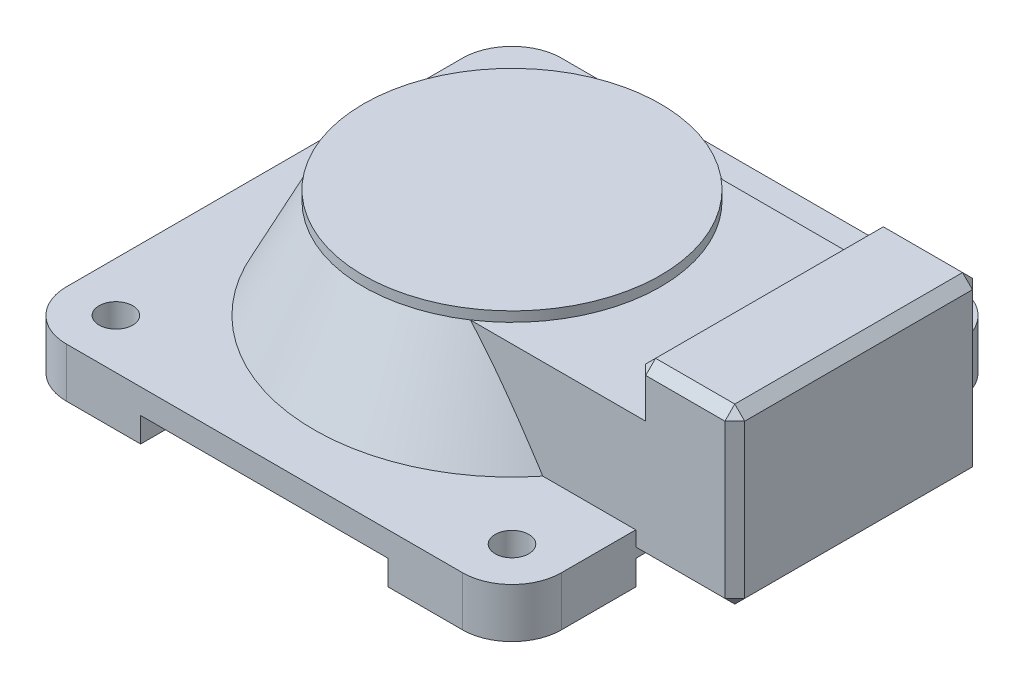
from build123d import *

# Parameters (mm, degrees)
SKETCH1_W             = 100
SKETCH1_H             = 100
BOSS_EXTRUDE1_DEPTH   = 10
SKETCH2_W             = 50
SKETCH2_H             = 10
CUT_EXTRUDE1_DEPTH    = 113.249721603
SKETCH3_W             = 50
SKETCH3_H             = 10
CUT_EXTRUDE2_DEPTH    = 113.249721603
FILLET1_R             = 10
SKETCH5_R             = 30
BOSS_EXTRUDE2_DEPTH   = 2
SKETCH6_W             = 50
SKETCH6_H             = 20
BOSS_EXTRUDE3_DEPTH   = 50
SKETCH7_W             = 50
SKETCH7_H             = 35
BOSS_EXTRUDE6_DEPTH   = 20
CHAMFER1_SIZE         = 2
M8_TAPPED_HOLE1_D     = 6.8
M8_TAPPED_HOLE1_DEPTH = 20.207073895
M8_TAPPED_HOLE1_TIP   = 2.042926105


with BuildPart() as part:
    # Sketch1 → Boss-Extrude1 (new body)
    with BuildSketch(Plane(origin=(0, 0, 0), x_dir=(1, 0, 0), z_dir=(0, 1, 0))):
        Rectangle(SKETCH1_W, SKETCH1_H)
    extrude(amount=BOSS_EXTRUDE1_DEPTH)

    # Sketch2 → Cut-Extrude1 (cut, through all)
    with BuildSketch(Plane.XY.offset(50)):
        Rectangle(SKETCH2_W, SKETCH2_H)
    extrude(amount=-CUT_EXTRUDE1_DEPTH, mode=Mode.SUBTRACT)

    # Sketch3 → Cut-Extrude2 (cut, through all)
    with BuildSketch(Plane(origin=(50, 0, 0), x_dir=(0, 0, -1), z_dir=(1, 0, 0))):
        Rectangle(SKETCH3_W, SKETCH3_H)
    extrude(amount=-CUT_EXTRUDE2_DEPTH, mode=Mode.SUBTRACT)

    # Fillet1
    fillet1_edges = [part.edges().sort_by_distance(p)[0] for p in [
        (50, 5, 50),
        (-50, 5, 50),
        (-50, 5, -50),
        (50, 5, -50),
    ]]
    fillet(fillet1_edges, radius=FILLET1_R)

    # Sketch4 → Revolve1 (revolve)
    with BuildSketch(Plane.XY):
        Polygon((0, 10), (0, 30), (30, 30), (40, 10), align=None)
    revolve(axis=Axis((0, 10, 0), (0, 1, 0)))

    # Sketch5 → Boss-Extrude2 (add)
    with BuildSketch(Plane(origin=(0, 30, 0), x_dir=(1, 0, 0), z_dir=(0, 1, 0))):
        with Locations(Location((0, 0, 0), (0, 0, 180))):
            Circle(SKETCH5_R)
    extrude(amount=BOSS_EXTRUDE2_DEPTH)

    # Sketch6 → Boss-Extrude3 (add)
    with BuildSketch(Plane(origin=(0, 0, 0), x_dir=(0, 0, -1), z_dir=(1, 0, 0))):
        with Locations((0, 20)):
            Rectangle(SKETCH6_W, SKETCH6_H)
    extrude(amount=BOSS_EXTRUDE3_DEPTH)

    # Sketch7 → Boss-Extrude6 (add)
    with BuildSketch(Plane(origin=(50, 0, 0), x_dir=(0, 0, -1), z_dir=(1, 0, 0))):
        with Locations((0, 22.5)):
            Rectangle(SKETCH7_W, SKETCH7_H)
    extrude(amount=BOSS_EXTRUDE6_DEPTH)

    # Chamfer1
    chamfer1_edges = [part.edges().sort_by_distance(p)[0] for p in [
        (70, 5, 0),
        (50, 40, 0),
        (60, 5, -25),
        (50, 35, -25),
        (60, 40, -25),
        (70, 22.5, -25),
        (70, 40, 0),
        (60, 5, 25),
        (70, 22.5, 25),
        (60, 40, 25),
        (50, 35, 25),
    ]]
    chamfer(chamfer1_edges, length=CHAMFER1_SIZE)

    # M8 Tapped Hole1
    with Locations(Plane(origin=(0, 10, 0), x_dir=(1, 0, 0), z_dir=(0, 1, 0))):
        with Locations((40, 40), (40, -40), (-40, -40), (-40, 40)):
            Hole(M8_TAPPED_HOLE1_D / 2, depth=M8_TAPPED_HOLE1_DEPTH)
            with Locations((0, 0, -(M8_TAPPED_HOLE1_DEPTH + M8_TAPPED_HOLE1_TIP / 2))):  # 118° drill point
                Cone(0, M8_TAPPED_HOLE1_D / 2, M8_TAPPED_HOLE1_TIP, mode=Mode.SUBTRACT)


solid = part.part
